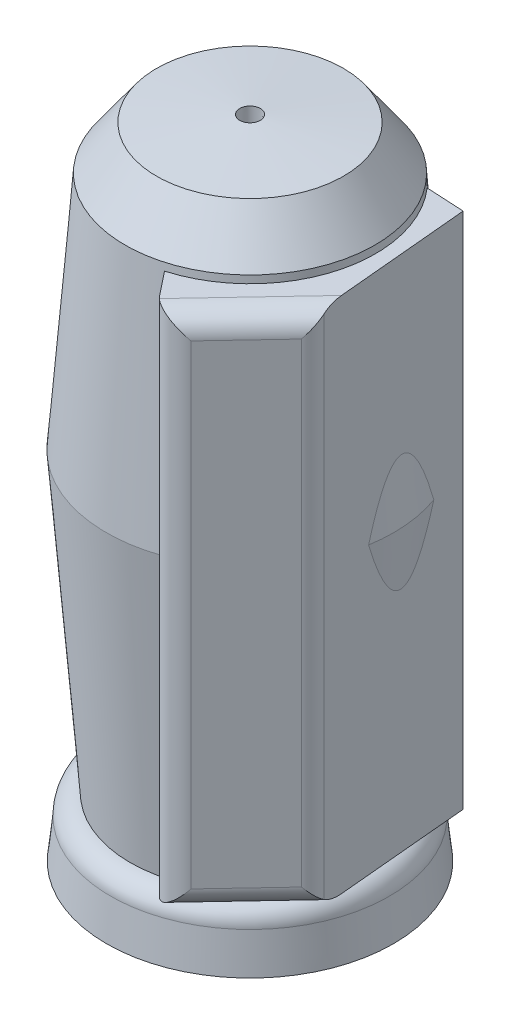
from build123d import *

# Parameters (mm, degrees)
BOSS_EXTRUDE1_DEPTH = 238
FILLET1_R           = 10


with BuildPart() as part:
    # Sketch2 → Revolve1 (revolve)
    with BuildSketch(Plane.XY, mode=Mode.PRIVATE) as revolve1_sk:
        with BuildLine():
            Line((-328.655679382, 26.621417908), (-366.845573795, 23.491008025))
            Line((-366.845573795, 23.491008025), (-381.297818843, 3.318082644))
            Line((-381.297818843, 3.318082644), (-389.923971527, -106.756034051))
            Line((-389.923971527, -106.756034051), (-379.0165134, -243.444434045))
            Line((-379.0165134, -243.444434045), (-328.318139163, -239.398806221))
            Line((-328.318139163, -239.398806221), (-328.561875404, -47.306824662))
            ThreePointArc((-328.561875404, -47.306824662), (-341.610700787, -42.948172925), (-331.054528121, -34.125650186))
            add(Edge.make_bspline(
                [(-343.396067048, -13.829139561), (-369.788894566, -3.962526401), (-364.86114786, -12.066545193), (-359.933401153, -20.170563985), (-331.054528121, -34.125650186)],
                knots=[2.07657219, 2.07657219, 2.07657219, 3.392364055, 3.392364055, 4.70815592, 4.70815592, 4.70815592], degree=2, weights=[1, 0.791280521, 1, 0.791280521, 1]))
            Line((-343.396067048, -13.829139561), (-328.632300571, 8.196246))
            Line((-328.632300571, 8.196246), (-328.655679382, 26.621417908))
        make_face()
    revolve(revolve1_sk.sketch.rotate(Axis((-323.917909898, -239.047676817, 0), (0, 1, 0)), 270), axis=Axis((-323.917909898, -239.047676817, 0), (0, 1, 0)))

    # Sketch3 → Boss-Extrude1 (add)
    with BuildSketch(Plane(origin=(0, 0, 0), x_dir=(1, 0, 0), z_dir=(0, 1, 0))):
        Polygon((-308.638521792, 39.575519818), (-263.153191414, 37.134281554), (-256.30786178, -37.667195745), (-291.882022487, -75.459531675), (-320.894913791, -38.858712112), (-298.848697668, -43.867323718), (-278.655979488, -19.734201659), (-273.594686567, 2.497883967), align=None)
    extrude(amount=-BOSS_EXTRUDE1_DEPTH)

    # Fillet1
    fillet1_edges = [part.edges().sort_by_distance(p)[0] for p in [
        (-291.882022487, -119, 75.459531675),
        (-274.094942134, -238, 56.56336371),
        (-256.30786178, -119, 37.667195745),
        (-274.094942134, 0, 56.56336371),
    ]]
    fillet(fillet1_edges, radius=FILLET1_R)


with BuildPart() as body_2:
    # Sketch5 → Revolve2 (revolve)
    with BuildSketch(Plane.XY, mode=Mode.PRIVATE) as revolve2_sk:
        with BuildLine():
            Line((-287.947541646, -243.444434045), (-268.819306396, -243.444434045))
            ThreePointArc((-268.819306396, -243.444434045), (-262.500398164, -246.061811534), (-259.883020675, -252.380719766))
            Line((-259.883020675, -252.380719766), (-258.037551648, -270.384607737))
            Line((-258.037551648, -270.384607737), (-289.850904646, -270.384607737))
            Line((-289.850904646, -270.384607737), (-287.947541646, -243.444434045))
        make_face()
    revolve(revolve2_sk.sketch.rotate(Axis((-323.917909898, 26.621417908, 0), (0, 1, 0)), 90), axis=Axis((-323.917909898, 26.621417908, 0), (0, 1, 0)))


solid = Compound([part.part, body_2.part])
